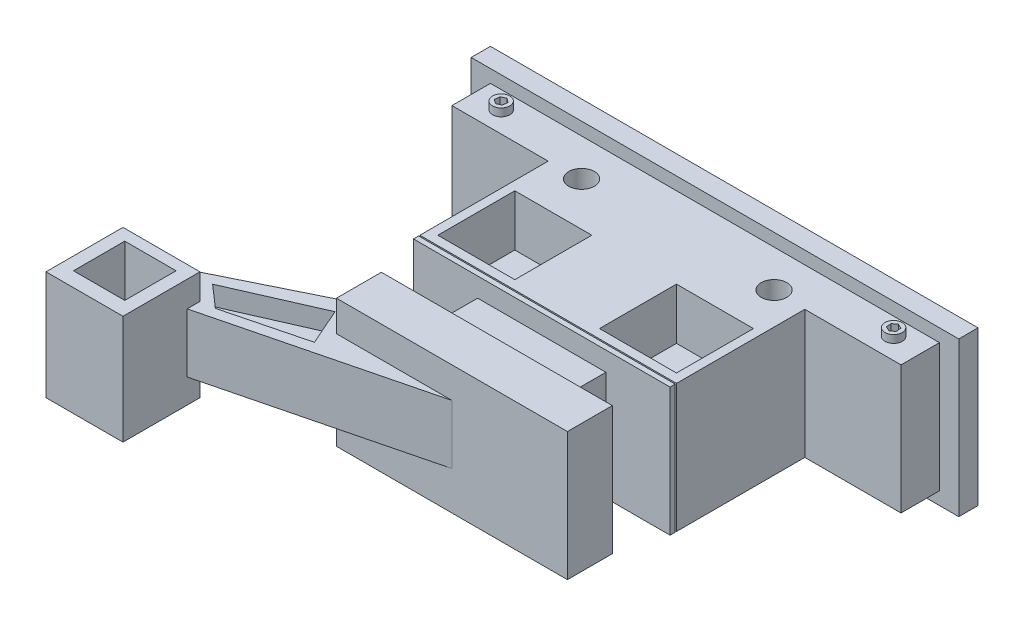
SolidWorks part; units mm, degrees
ref_plane "Front Plane" through (0, 0, 0) normal (0, 0, 1) x (1, 0, 0)
ref_plane "Top Plane" through (0, 0, 0) normal (0, 1, 0) x (1, 0, 0)
ref_plane "Right Plane" through (0, 0, 0) normal (1, 0, 0) x (0, 0, -1)
other "Configuration Table"
sketch "Sketch1" plane through (0, 0, 0) normal (0, 1, 0) x (1, 0, 0)
  line L0 (0, 0) -> (0, 35)
  line L1 (0, 35) -> (40, 35)
  line L2 (40, 35) -> (40, 75)
  line L3 (40, 75) -> (-10, 75)
  line L4 (-10, 75) -> (-10, 175)
  line L5 (-10, 175) -> (-85, 175)
  line L6 (-85, 175) -> (-85, 220)
  line L7 (-85, 220) -> (265, 220)
  line L8 (265, 220) -> (265, 175)
  line L9 (265, 175) -> (190, 175)
  line L10 (190, 175) -> (190, 75)
  line L11 (190, 75) -> (140, 75)
  line L12 (140, 75) -> (140, 35)
  line L13 (140, 35) -> (180, 35)
  line L14 (180, 35) -> (180, 0)
  line L15 (180, 0) -> (0, 0)
  dimension "D1" = 220
  dimension "D2" = 40
  dimension "D3" = 350
  dimension "D4" = 75
  dimension "D5" = 75
  dimension "D6" = 50
  dimension "D7" = 50
  dimension "D8" = 40
  dimension "D9" = 35
  dimension "D10" = 40
  dimension "D11" = 40
  dimension "D12" = 35
  dimension "D13" = 100
  dimension "D14" = 100
extrude "Boss-Extrude1" add sketch "Sketch1" along normal blind 100
sketch "Sketch2" plane through (0, 100, 0) normal (0, 1, 0) x (1, 0, 0)
  line L0 (-10, 75) -> (40, 75) construction
  line L1 (-3, 82) -> (57, 82)
  line L2 (-3, 82) -> (-3, 142)
  line L3 (-3, 142) -> (57, 142)
  line L4 (57, 82) -> (57, 142)
  line L5 (183, 82) -> (123, 82)
  line L6 (183, 82) -> (183, 142)
  line L7 (183, 142) -> (123, 142)
  line L8 (123, 82) -> (123, 142)
  line L9 (-10, 175) -> (-10, 75) construction
  line L10 (190, 75) -> (190, 175) construction
  line L11 (140, 75) -> (190, 75) construction
  dimension "D1" = 60
  dimension "D2" = 60
  dimension "D3" = 60
  dimension "D4" = 60
  dimension "D5" = 7
  dimension "D6" = 7
  dimension "D7" = 7
  dimension "D8" = 7
extrude "Cut-Extrude1" cut sketch "Sketch2" against normal blind 40
ref_plane "Plane1" through (0, 50, 0) normal (0, 1, 0) x (1, 0, 0)
mirror "Mirror1" about plane through (0, 50, 0) normal (0, 1, 0) of "Cut-Extrude1"
sketch "Sketch3" plane through (0, 100, 0) normal (0, 1, 0) x (1, 0, 0)
  line L1 (40, 35) -> (140, 35)
  line L2 (40, 35) -> (40, 75)
  line L3 (40, 75) -> (140, 75)
  line L4 (140, 35) -> (140, 75)
extrude "Cut-Extrude2" cut sketch "Sketch3" against normal blind 15
mirror "Mirror2" about plane through (0, 50, 0) normal (0, 1, 0) of "Cut-Extrude2"
sketch "Sketch4" plane through (0, 0, -220) normal (0, 0, -1) x (-1, 0, 0)
  line L0 (-265, 100) -> (85, 0) construction
  line L2 (-280, 110) -> (100, 110)
  line L3 (-280, 110) -> (-280, -10)
  line L4 (-280, -10) -> (100, -10)
  line L5 (100, 110) -> (100, -10)
  line L6 (-280, 110) -> (100, -10) construction
  line L7 (-280, -10) -> (100, 110) construction
  point P4 (-90, 50)
  dimension "D1" = 120
  dimension "D2" = 380
extrude "Boss-Extrude2" add sketch "Sketch4" against normal blind 15
sketch "Sketch5" plane through (0, 0, -82) normal (0, 0, -1) x (-1, 0, 0)
  line L0 (3, 40) -> (3, 0) construction
  line L1 (3, 0) -> (-57, 0) construction
  line L3 (-7.3846, 10.3644) -> (-6.7758, 12.5811)
  line L4 (-6.7758, 12.5811) -> (-8.3912, 14.2168)
  line L5 (-8.3912, 14.2168) -> (-10.6154, 13.6356)
  line L6 (-10.6154, 13.6356) -> (-11.2242, 11.4189)
  line L7 (-11.2242, 11.4189) -> (-9.6088, 9.7832)
  line L8 (-9.6088, 9.7832) -> (-7.3846, 10.3644)
  circle A0 centre (-9, 12) radius 4
  circle A1 centre (-9, 12) radius 1.9909 construction
  dimension "D1" = 8
  dimension "D3" = 12
  dimension "D2" = 12
extrude "Boss-Extrude3" add sketch "Sketch5" along normal blind 4
ref_plane "Plane2" through (90, 0, 0) normal (-1, 0, 0) x (0, 0, 1)
mirror "Mirror3" about plane through (90, 0, 0) normal (-1, 0, 0) of "Boss-Extrude3"
mirror "Mirror4" about plane through (0, 50, 0) normal (0, 1, 0) of "Mirror3", "Boss-Extrude3"
sketch "Sketch6" plane through (0, 0, -75) normal (0, 0, 1) x (1, 0, 0)
  line L0 (90, 55) -> (90, -55) construction
  line L1 (-6.8498, 96.8628) -> (186.8498, 96.8628)
  line L2 (-6.8498, 96.8628) -> (-6.8498, 3.1372)
  line L3 (-6.8498, 3.1372) -> (186.8498, 3.1372)
  line L4 (186.8498, 96.8628) -> (186.8498, 3.1372)
  line L5 (-6.8498, 96.8628) -> (186.8498, 3.1372) construction
  line L6 (-6.8498, 3.1372) -> (186.8498, 96.8628) construction
  line L7 (71.5, 50) -> (-71.5, 50) construction
  point P0 (90, 50)
extrude "Boss-Extrude4" add sketch "Sketch6" along normal blind 1
sketch "Sketch7" plane through (0, 0, -74) normal (0, 0, 1) x (1, 0, 0)
  line L0 (90, 55) -> (90, -55) construction
  line L1 (-10, 100) -> (190, 100)
  line L2 (-10, 100) -> (-10, 0)
  line L3 (-10, 0) -> (190, 0)
  line L4 (190, 100) -> (190, 0)
  line L5 (-10, 100) -> (190, 0) construction
  line L6 (-10, 0) -> (190, 100) construction
  line L7 (71.5, 50) -> (-71.5, 50) construction
  point P0 (90, 50)
extrude "Boss-Extrude5" add sketch "Sketch7" along normal blind 4
sketch "Sketch8" plane through (140, 0, 0) normal (1, 0, 0) x (0, 0, -1)
  line L1 (40.6133, 67.4954) -> (65.3688, 67.4954)
  line L2 (40.6133, 67.4954) -> (40.6133, 32.0285)
  line L3 (40.6133, 32.0285) -> (65.3688, 32.0285)
  line L4 (65.3688, 67.4954) -> (65.3688, 32.0285)
  line L5 (40.6133, 67.4954) -> (65.3688, 32.0285) construction
  line L6 (40.6133, 32.0285) -> (65.3688, 67.4954) construction
  point P0 (52.991, 49.762)
extrude "Cut-Extrude3" cut sketch "Sketch8" against normal up to next
sketch "Sketch9" plane through (0, 0, -35) normal (0, 0, -1) x (-1, 0, 0)
  line L0 (-180, 100) -> (-180, 0) construction
  line L1 (-180, 100) -> (0, 100) construction
  circle A0 centre (-168, 88) radius 7.5
  dimension "D1" = 15
  dimension "D2" = 12
  dimension "D3" = 12
extrude "Boss-Extrude6" add sketch "Sketch9" along normal blind 1.5
sketch "Sketch10" plane through (0, 0, -36.5) normal (0, 0, -1) x (-1, 0, 0)
  line L1 (-169.0831, 85.4589) -> (-166.3409, 85.7914)
  line L2 (-166.3409, 85.7914) -> (-165.2578, 88.3325)
  line L3 (-165.2578, 88.3325) -> (-166.9169, 90.5411)
  line L4 (-166.9169, 90.5411) -> (-169.6591, 90.2086)
  line L5 (-169.6591, 90.2086) -> (-170.7422, 87.6675)
  line L6 (-170.7422, 87.6675) -> (-169.0831, 85.4589)
  circle A0 centre (-168, 88) radius 5.0501
  circle A1 centre (-168, 88) radius 2.3922 construction
extrude "Boss-Extrude7" add sketch "Sketch10" along normal blind 5
mirror "Mirror5" about plane through (90, 0, 0) normal (-1, 0, 0) of "Boss-Extrude6", "Boss-Extrude7"
mirror "Mirror6" about plane through (0, 50, 0) normal (0, 1, 0) of "Mirror5", "Boss-Extrude6", "Boss-Extrude7"
sketch "Sketch11" plane through (0, 100, 0) normal (0, 1, 0) x (1, 0, 0)
  line L0 (190, 75) -> (190, 175) construction
  circle A0 centre (15, 176.0407) radius 10
  circle A1 centre (165, 176.0407) radius 10
  dimension "D1" = 20
  dimension "D2" = 20
  dimension "D3" = 25
  dimension "D4" = 25
extrude "Cut-Extrude4" cut sketch "Sketch11" against normal up to next
sketch "Sketch12" plane through (0, 100, 0) normal (0, 1, 0) x (1, 0, 0)
  line L1 (-59.6489, 188.9628) -> (-59.2445, 192.9893)
  line L2 (-59.2445, 192.9893) -> (-62.5293, 195.3527)
  line L3 (-62.5293, 195.3527) -> (-66.2186, 193.6897)
  line L4 (-66.2186, 193.6897) -> (-66.623, 189.6632)
  line L5 (-66.623, 189.6632) -> (-63.3381, 187.2997)
  line L6 (-63.3381, 187.2997) -> (-59.6489, 188.9628)
  circle A0 centre (-62.9337, 191.3262) radius 6.7128
  circle A1 centre (-62.9337, 191.3262) radius 3.5046 construction
extrude "Boss-Extrude8" add sketch "Sketch12" along normal blind 6
mirror "Mirror7" about plane through (90, 0, 0) normal (-1, 0, 0) of "Boss-Extrude8"
mirror "Mirror8" about plane through (0, 50, 0) normal (0, 1, 0) of "Mirror7", "Boss-Extrude8"
sketch "Sketch13" plane through (0, 50, 0) normal (0, 1, 0) x (1, 0, 0)
  line L0 (0, 0) -> (-85, 0) construction
  line L1 (-85, 0) -> (-85, -40) construction
  line L3 (-135, -31.3837) -> (-135, -91.3837)
  line L4 (-135, -91.3837) -> (-75, -91.3837)
  line L5 (-75, -91.3837) -> (-75, -41.3837)
  line L6 (-75, -41.3837) -> (90, 0)
  line L9 (-135, -31.3837) -> (0, 35)
  line L10 (-85, -40) -> (-125, -40)
  line L11 (-85, -40) -> (-85, -80)
  line L12 (-85, -80) -> (-125, -80)
  line L13 (-125, -40) -> (-125, -80)
  line L14 (0, 35) -> (90, 0)
  dimension "D1" = 85
  dimension "D2" = 40
  dimension "D3" = 50
  dimension "D4" = 60
  dimension "D5" = 60
  dimension "D6" = 10
  dimension "D7" = 40
  dimension "D8" = 40
extrude "Boss-Extrude9" add sketch "Sketch13" along normal blind 26 and the other way blind 20
sketch "Sketch14" plane through (0, 76, 0) normal (0, 1, 0) x (1, 0, 0)
  line L1 (-125, -40) -> (-85, -40)
  line L2 (-125, -40) -> (-125, -80)
  line L3 (-125, -80) -> (-85, -80)
  line L4 (-85, -40) -> (-85, -80)
  line L5 (-135, -31.3837) -> (-75, -31.3837)
  line L6 (-135, -31.3837) -> (-135, -91.3837)
  line L7 (-135, -91.3837) -> (-75, -91.3837)
  line L8 (-75, -31.3837) -> (-75, -91.3837)
extrude "Boss-Extrude10" add sketch "Sketch14" along normal blind 20 and the other way blind 65
sketch "Sketch15" plane through (0, 76, 0) normal (0, 1, 0) x (1, 0, 0)
  line L0 (-81.724, -14.8101) -> (-15.4357, 14.3133)
  line L1 (-15.4357, 14.3133) -> (-2.8299, -14.3789)
  line L2 (-2.8299, -14.3789) -> (-64.323, -30.0657)
  line L3 (-64.323, -30.0657) -> (-81.724, -14.8101)
extrude "Cut-Extrude5" cut sketch "Sketch15" against normal blind 15
mirror "Mirror11" about plane through (0, 50, 0) normal (0, 1, 0) of "Cut-Extrude5"
